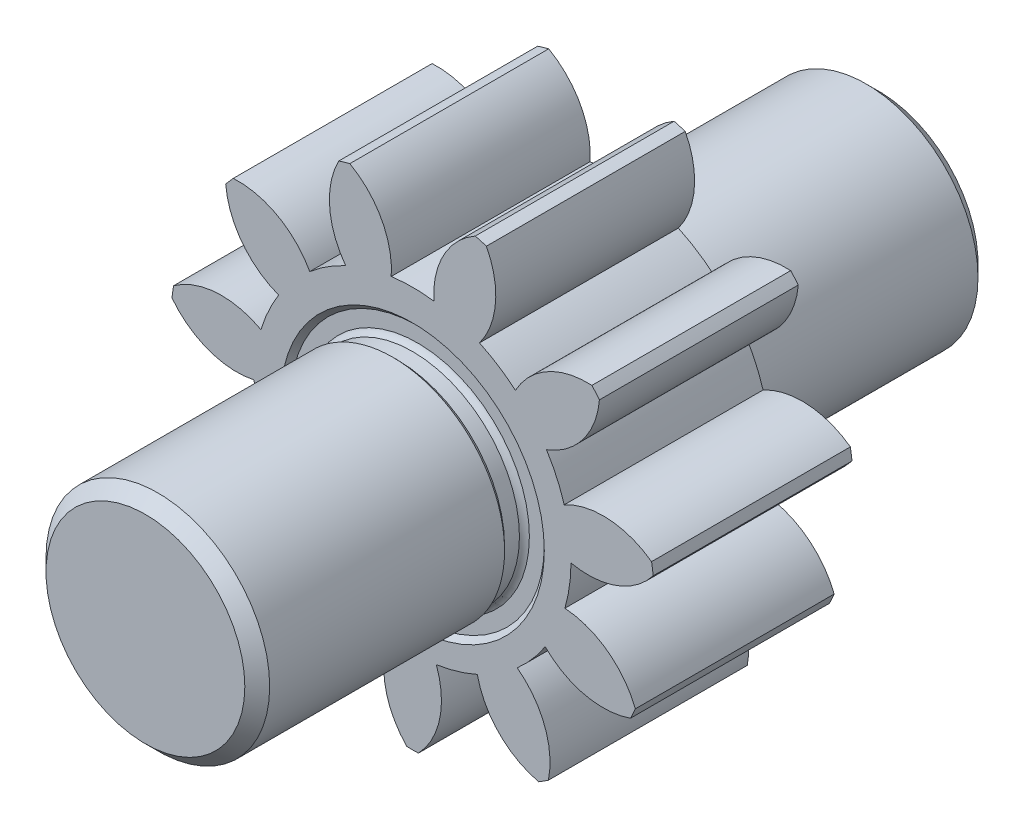
SolidWorks part; units mm, degrees
ref_plane "前视基准面" through (0, 0, 0) normal (0, 0, 1) x (1, 0, 0)
ref_plane "上视基准面" through (0, 0, 0) normal (0, 1, 0) x (1, 0, 0)
ref_plane "右视基准面" through (0, 0, 0) normal (1, 0, 0) x (0, 0, -1)
sketch "草图2" plane through (0, 0, 0) normal (0, 0, 1) x (1, 0, 0)
  arc A0 (-17.5397, -8.1889) -> (-10.6725, -6.6417) centre (-15.3333, -1.9687) ccw
  arc A1 (-10.6725, -6.6417) -> (-8.4217, -9.2393) centre (0, 0.3321) ccw
  arc A2 (-8.4217, -9.2393) -> (-10.9305, -15.8164) centre (-4.4595, -14.5176) ccw
  arc A3 (-10.9305, -15.8164) -> (-10.1485, -16.3189) centre (0, 0.3321) ccw
  arc A4 (-10.1485, -16.3189) -> (-5.2079, -11.3046) centre (-11.6553, -9.8932) ccw
  arc A5 (-5.2079, -11.3046) -> (-1.9101, -12.273) centre (0, 0.3321) ccw
  arc A6 (-1.9101, -12.273) -> (-0.4648, -19.1623) centre (4.2768, -14.5713) ccw
  arc A7 (-0.4648, -19.1623) -> (0.4648, -19.1623) centre (0, 0.3321) ccw
  arc A8 (0.4648, -19.1623) -> (1.9101, -12.273) centre (-4.2768, -14.5713) ccw
  arc A9 (1.9101, -12.273) -> (5.2079, -11.3046) centre (0, 0.3321) ccw
  arc A10 (5.2079, -11.3046) -> (10.1485, -16.3189) centre (11.6553, -9.8932) ccw
  arc A11 (10.1485, -16.3189) -> (10.9305, -15.8164) centre (0, 0.3321) ccw
  arc A12 (10.9305, -15.8164) -> (8.4217, -9.2393) centre (4.4595, -14.5176) ccw
  arc A13 (8.4217, -9.2393) -> (10.6725, -6.6417) centre (0, 0.3321) ccw
  arc A14 (10.6725, -6.6417) -> (17.5397, -8.1889) centre (15.3333, -1.9687) ccw
  arc A15 (17.5397, -8.1889) -> (17.9259, -7.3434) centre (0, 0.3321) ccw
  arc A16 (17.9259, -7.3434) -> (12.2595, -3.1667) centre (11.78, -9.7493) ccw
  arc A17 (12.2595, -3.1667) -> (12.7486, 0.2354) centre (0, 0.3321) ccw
  arc A18 (12.7486, 0.2354) -> (19.3622, 2.6465) centre (14.1431, 6.6864) ccw
  arc A19 (19.3622, 2.6465) -> (19.2299, 3.5665) centre (0, 0.3321) ccw
  arc A20 (19.2299, 3.5665) -> (12.205, 4.0167) centre (15.3604, -1.7802) ccw
  arc A21 (12.205, 4.0167) -> (10.7771, 7.1432) centre (0, 0.3321) ccw
  arc A22 (10.7771, 7.1432) -> (15.0373, 12.7471) centre (8.4625, 13.324) ccw
  arc A23 (15.0373, 12.7471) -> (14.4286, 13.4495) centre (0, 0.3321) ccw
  arc A24 (14.4286, 13.4495) -> (8.2754, 10.0303) centre (14.064, 6.8596) ccw
  arc A25 (8.2754, 10.0303) -> (5.384, 11.8885) centre (0, 0.3321) ccw
  arc A26 (5.384, 11.8885) -> (5.9382, 18.906) centre (0.0952, 15.8368) ccw
  arc A27 (5.9382, 18.906) -> (5.0463, 19.1679) centre (0, 0.3321) ccw
  arc A28 (5.0463, 19.1679) -> (1.7185, 12.9648) centre (8.3023, 13.4269) ccw
  arc A29 (1.7185, 12.9648) -> (-1.7185, 12.9648) centre (0, 0.3321) ccw
  arc A30 (-1.7185, 12.9648) -> (-5.0463, 19.1679) centre (-8.3023, 13.4269) ccw
  arc A31 (-5.0463, 19.1679) -> (-5.9382, 18.906) centre (0, 0.3321) ccw
  arc A32 (-5.9382, 18.906) -> (-5.384, 11.8885) centre (-0.0952, 15.8368) ccw
  arc A33 (-5.384, 11.8885) -> (-8.2754, 10.0303) centre (0, 0.3321) ccw
  arc A34 (-8.2754, 10.0303) -> (-14.4286, 13.4495) centre (-14.064, 6.8596) ccw
  arc A35 (-14.4286, 13.4495) -> (-15.0373, 12.7471) centre (0, 0.3321) ccw
  arc A36 (-15.0373, 12.7471) -> (-10.7771, 7.1432) centre (-8.4625, 13.324) ccw
  arc A37 (-10.7771, 7.1432) -> (-12.205, 4.0167) centre (0, 0.3321) ccw
  arc A38 (-12.205, 4.0167) -> (-19.2299, 3.5665) centre (-15.3604, -1.7802) ccw
  arc A39 (-19.2299, 3.5665) -> (-19.3622, 2.6465) centre (0, 0.3321) ccw
  arc A40 (-19.3622, 2.6465) -> (-12.7486, 0.2354) centre (-14.1431, 6.6864) ccw
  arc A41 (-12.7486, 0.2354) -> (-12.2595, -3.1667) centre (0, 0.3321) ccw
  arc A42 (-12.2595, -3.1667) -> (-17.9259, -7.3434) centre (-11.78, -9.7493) ccw
  arc A43 (-17.9259, -7.3434) -> (-17.5397, -8.1889) centre (0, 0.3321) ccw
extrude "凸台-拉伸1" add sketch "草图2" along normal blind 16
sketch "草图3" plane through (0, 0, 16) normal (0, 0, 1) x (1, 0, 0)
  circle A0 centre (0, 0) radius 9
  dimension "D1" = 18
extrude "凸台-拉伸2" add sketch "草图3" along normal blind 21.5
sketch "草图4" plane through (0, 0, 0) normal (1, 0, 0) x (0, 0, -1)
  line L0 (-17.6, 8.9996) -> (-17.2, 8.5996)
  line L1 (-17.2, 8.5996) -> (-16, 8.5996)
  line L2 (-16, 9) -> (-16, -9) construction
  line L3 (-17.6, 8.9996) -> (-17.6, 10.5996)
  line L4 (-17.6, 10.5996) -> (-16, 10.5996)
  line L5 (-16, 18.906) -> (-16, 11.8885) construction
  line L6 (-16, 10.5996) -> (-15.6, 10.1996)
  line L7 (-15.6, 10.1996) -> (-15.6, 8.9996)
  line L8 (-16, 12.7471) -> (-16, 7.1432) construction
  arc A0 (-15.6, 8.9996) -> (-16, 8.5996) centre (-16.3292, 9.3288) cw
  point P12 (-20.7587, 10.6326)
  point P13 (-20.7638, 10.5033)
  point P14 (-20.7453, 8.925)
  point P15 (-20.7798, 10.61)
  point P16 (-20.7981, 8.9996)
  point P19 (-15.6, 8.9996)
  point P20 (-17.6, 8.9996)
  dimension "D6" = 0.8
  dimension "D1" = 135
  dimension "D2" = 2
  dimension "D3" = 0.4
  dimension "D4" = 0.4
  dimension "D5" = 2
revolve "切除-旋转1" cut sketch "草图4" angle 360 about axis through (0, 0, 37.5) along (0, 0, -1)
ref_plane "基准面1" through (0, 0, 8) normal (0, 0, 1) x (1, 0, 0)
mirror "镜向1" about plane through (0, 0, 8) normal (0, 0, 1) of "切除-旋转1", "凸台-拉伸2"
chamfer "倒角1" distance 1 angle 45 2 edges at (9, 0, -21.5) (9, 0, 37.5)
